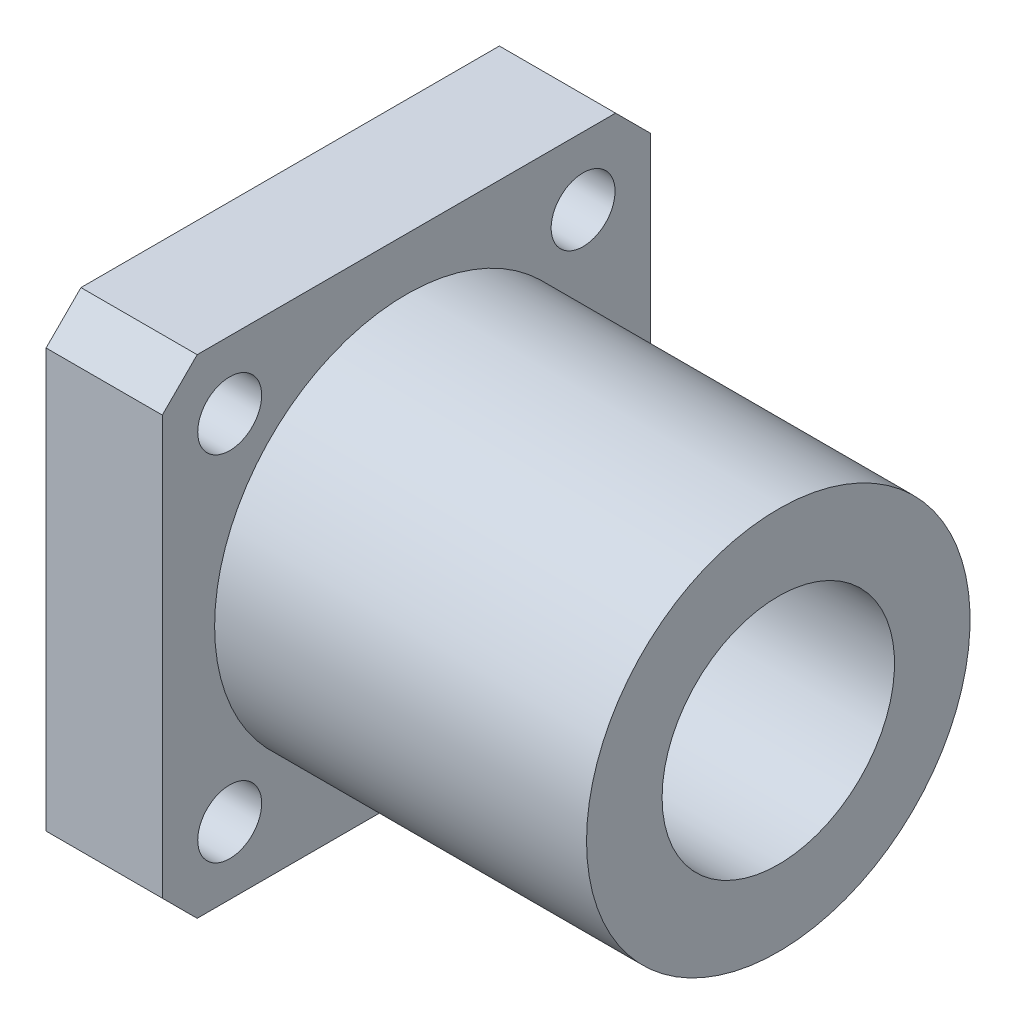
SolidWorks part; units mm, degrees
ref_plane "Front Plane" through (0, 0, 0) normal (0, 0, 1) x (1, 0, 0)
ref_plane "Top Plane" through (0, 0, 0) normal (0, 1, 0) x (1, 0, 0)
ref_plane "Right Plane" through (0, 0, 0) normal (1, 0, 0) x (0, 0, -1)
sketch "Sketch1" plane through (0, 0, 0) normal (1, 0, 0) x (0, 0, -1)
  line L0 (-21, 21) -> (-21, -21)
  line L1 (21, -21) -> (21, 21)
  line L2 (0, 0) -> (-21, 0) construction
  line L3 (21, 21) -> (-21, 21)
  line L4 (21, -21) -> (-21, -21)
  line L5 (0, 0) -> (0, 21) construction
  dimension "D1" = 42
extrude "Boss-Extrude1" add sketch "Sketch1" along normal blind 10
sketch "Sketch2" plane through (10, 0, 0) normal (1, 0, 0) x (0, 0, -1)
  circle A0 centre (0, 0) radius 16.5
  dimension "D1" = 33
extrude "Boss-Extrude2" add sketch "Sketch2" along normal blind 32
hole_wizard "Ø5.5 (5.5) Diameter Hole1" positions "Sketch4" profile "Sketch3" hole size "Ø5.5" standard "GB" end condition through all
sketch "Sketch4" plane through (0, 0, 0) normal (-1, 0, 0) x (0, 0, 1)
  line L1 (15.2028, 15.2028) -> (-15.2028, 15.2028) construction
  line L2 (15.2028, 15.2028) -> (15.2028, -15.2028) construction
  line L3 (15.2028, -15.2028) -> (-15.2028, -15.2028) construction
  line L4 (-15.2028, 15.2028) -> (-15.2028, -15.2028) construction
  line L5 (15.2028, 0) -> (0, 0) construction
  line L6 (0, 0) -> (0, 15.2028) construction
  circle A0 centre (0, 0) radius 21.5 construction
  point P1 (-15.2028, 15.2028)
  point P2 (15.2028, 15.2028)
  point P3 (15.2028, -15.2028)
  point P5 (-15.2028, -15.2028)
  dimension "D1" = 43
sketch "Sketch3" plane through (0, 15.2028, -15.2028) normal (0, 1, 0) x (0, 0, 1)
  line L0 (0, 0) -> (0, 42)
  line L1 (0, 42) -> (2.75, 42)
  line L2 (2.75, 42) -> (2.75, 0)
  line L5 (2.75, 0) -> (0, 0)
  line L11 (0, -6.35) -> (0, 107.95) construction
  dimension "通孔孔直径" = 5.5
  dimension "通孔孔深度" = 42
sketch "Sketch7" plane through (0, 0, 0) normal (-1, 0, 0) x (0, 0, 1)
  circle A0 centre (0, 0) radius 10
  dimension "D1" = 20
extrude "Cut-Extrude1" cut sketch "Sketch7" against normal through all
chamfer "Chamfer1" distance 3 angle 45 4 edges at (5, 21, -21) (5, -21, -21) (5, -21, 21) (5, 21, 21)
